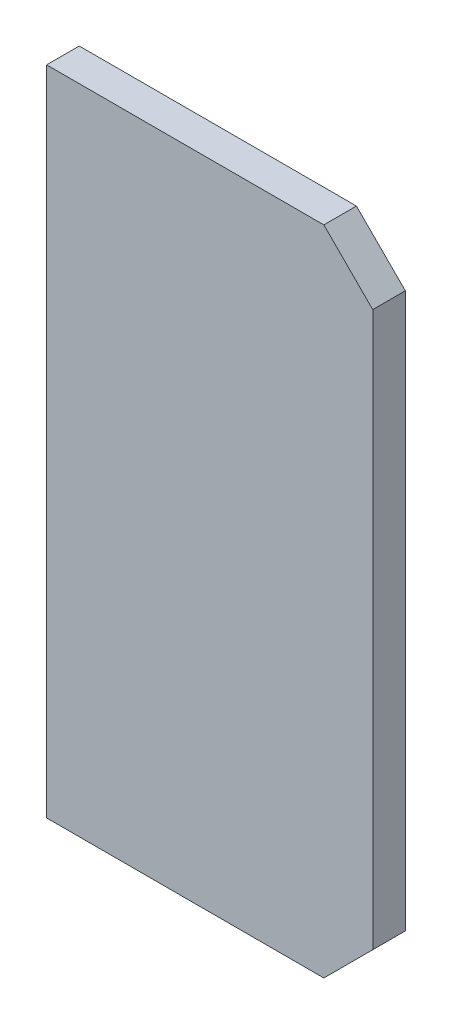
SolidWorks part; units mm, degrees
material "XRAAT"
ref_plane "前视基准面" through (0, 0, 0) normal (0, 0, 1) x (1, 0, 0)
ref_plane "上视基准面" through (0, 0, 0) normal (0, 1, 0) x (1, 0, 0)
ref_plane "右视基准面" through (0, 0, 0) normal (1, 0, 0) x (0, 0, -1)
sketch "草图1" plane through (0, 0, 0) normal (0, 0, 1) x (1, 0, 0)
  line L0 (0, 0) -> (0, 150)
  line L1 (0, 150) -> (46, 200)
  line L2 (46, 200) -> (100, 200)
  line L3 (100, 200) -> (100, 0)
  line L4 (100, 0) -> (0, 0)
  dimension "D1" = 100
  dimension "D2" = 150
  dimension "D3" = 200
  dimension "D4" = 54
extrude "凸台-拉伸1" add sketch "草图1" along normal mid plane 10
chamfer "倒角1" distance 15 angle 45 2 edges at (100, 0, 0) (100, 200, 0)
sketch "草图2" plane through (0, 0, 5) normal (0, 0, 1) x (1, 0, 0)
  line L0 (0, 150) -> (0, 200)
  line L1 (0, 200) -> (46, 200)
  line L2 (46, 200) -> (0, 150) construction
  line L3 (46, 200) -> (0, 150)
extrude "凸台-拉伸2" add sketch "草图2" against normal up to surface (10 mm away) up to face at (59.4286, 107.1429, -5)
